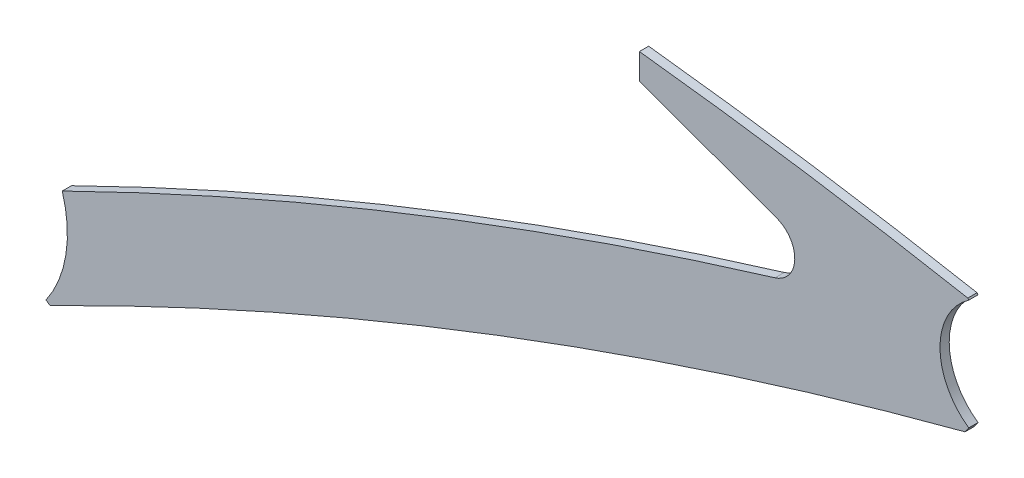
from build123d import *

# Parameters (mm, degrees)
BOSS_EXTRUDE1_DEPTH = 10


with BuildPart() as part:
    # Sketch1 → Boss-Extrude1 (new body)
    with BuildSketch(Plane.XY):
        with BuildLine():
            ThreePointArc((893.221093202, 341.53568212), (914.498906919, 369.426423756), (894.770629974, 398.433904074))
            Line((894.770629974, 398.433904074), (746.5, 452.4))
            Line((746.5, 452.4), (746.5, 480.1))
            ThreePointArc((746.5, 480.1), (924.530143798, 456.633232126), (1101.599381764, 426.768432422))
            Line((1101.599381764, 426.768432422), (1102.628920146, 425.298099233))
            ThreePointArc((1102.628920146, 425.298099233), (1071.5, 365.5), (1102.628920146, 305.701900767))
            Line((1102.628920146, 305.701900767), (1098.632098759, 299.99384827))
            ThreePointArc((1098.632098759, 299.99384827), (593.965714202, 137.948571105), (109.234583042, -76.486878479))
            Line((109.234583042, -76.486878479), (104.851461669, -73.417783853))
            ThreePointArc((104.851461669, -73.417783853), (126.422272258, -20.035195957), (122.413865115, 37.401144736))
            ThreePointArc((122.413865115, 37.401144736), (501.640075089, 205.12460213), (893.221093202, 341.53568212))
        make_face()
    extrude(amount=BOSS_EXTRUDE1_DEPTH)


solid = part.part
